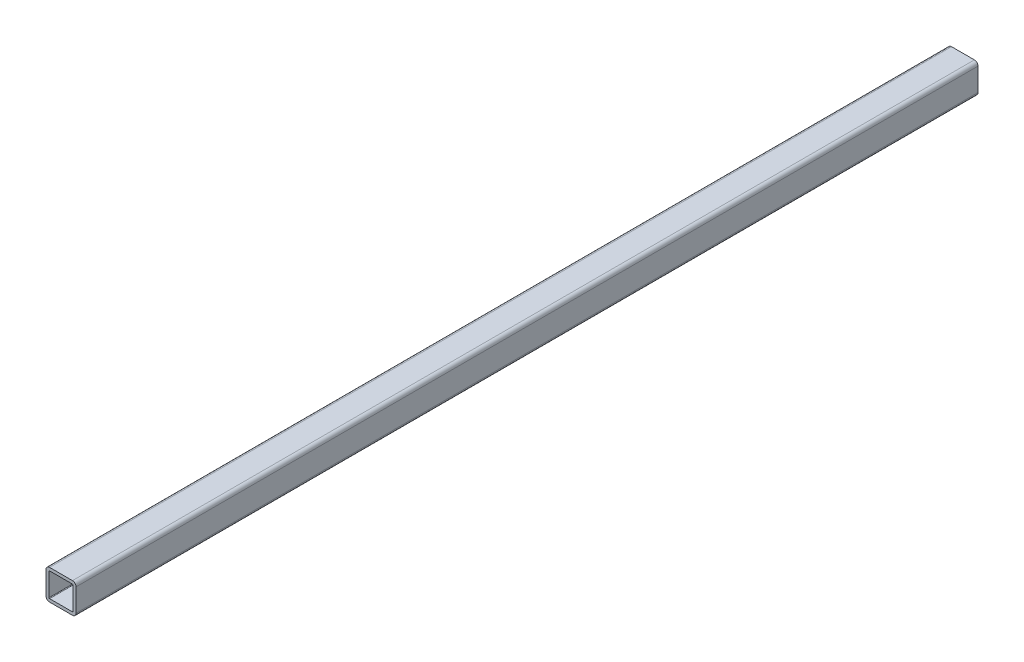
SolidWorks part; units mm, degrees
material "Q235B"
ref_plane "Front Plane" through (0, 0, 0) normal (0, 0, 1) x (1, 0, 0)
ref_plane "Top Plane" through (0, 0, 0) normal (0, 1, 0) x (1, 0, 0)
ref_plane "Right Plane" through (0, 0, 0) normal (1, 0, 0) x (0, 0, -1)
sketch "Sketch1" plane through (0, 0, 0) normal (0, 0, 1) x (1, 0, 0)
  line L0 (6, 45) -> (44, 45)
  line L1 (6, 0) -> (44, 0)
  line L2 (0, 6) -> (0, 44)
  line L3 (6, 50) -> (44, 50)
  line L4 (50, 6) -> (50, 44)
  line L5 (45, 6) -> (45, 44)
  line L6 (6, 5) -> (44, 5)
  line L7 (5, 6) -> (5, 44)
  arc A0 (6, 0) -> (0, 6) centre (6, 6) cw
  arc A1 (44, 0) -> (50, 6) centre (44, 6) ccw
  arc A2 (44, 50) -> (50, 44) centre (44, 44) cw
  arc A3 (0, 44) -> (6, 50) centre (6, 44) cw
  arc A4 (5, 44) -> (6, 45) centre (6, 44) cw
  arc A5 (44, 45) -> (45, 44) centre (44, 44) cw
  arc A6 (44, 5) -> (45, 6) centre (44, 6) ccw
  arc A7 (6, 5) -> (5, 6) centre (6, 6) cw
  point P7 (0, 0)
  point P12 (50, 50)
  point P15 (0, 50)
  dimension "D3" = 6
  dimension "D1" = 50
  dimension "D2" = 50
  dimension "D4" = 5
extrude "Boss-Extrude1" add sketch "Sketch1" along normal blind 1500
